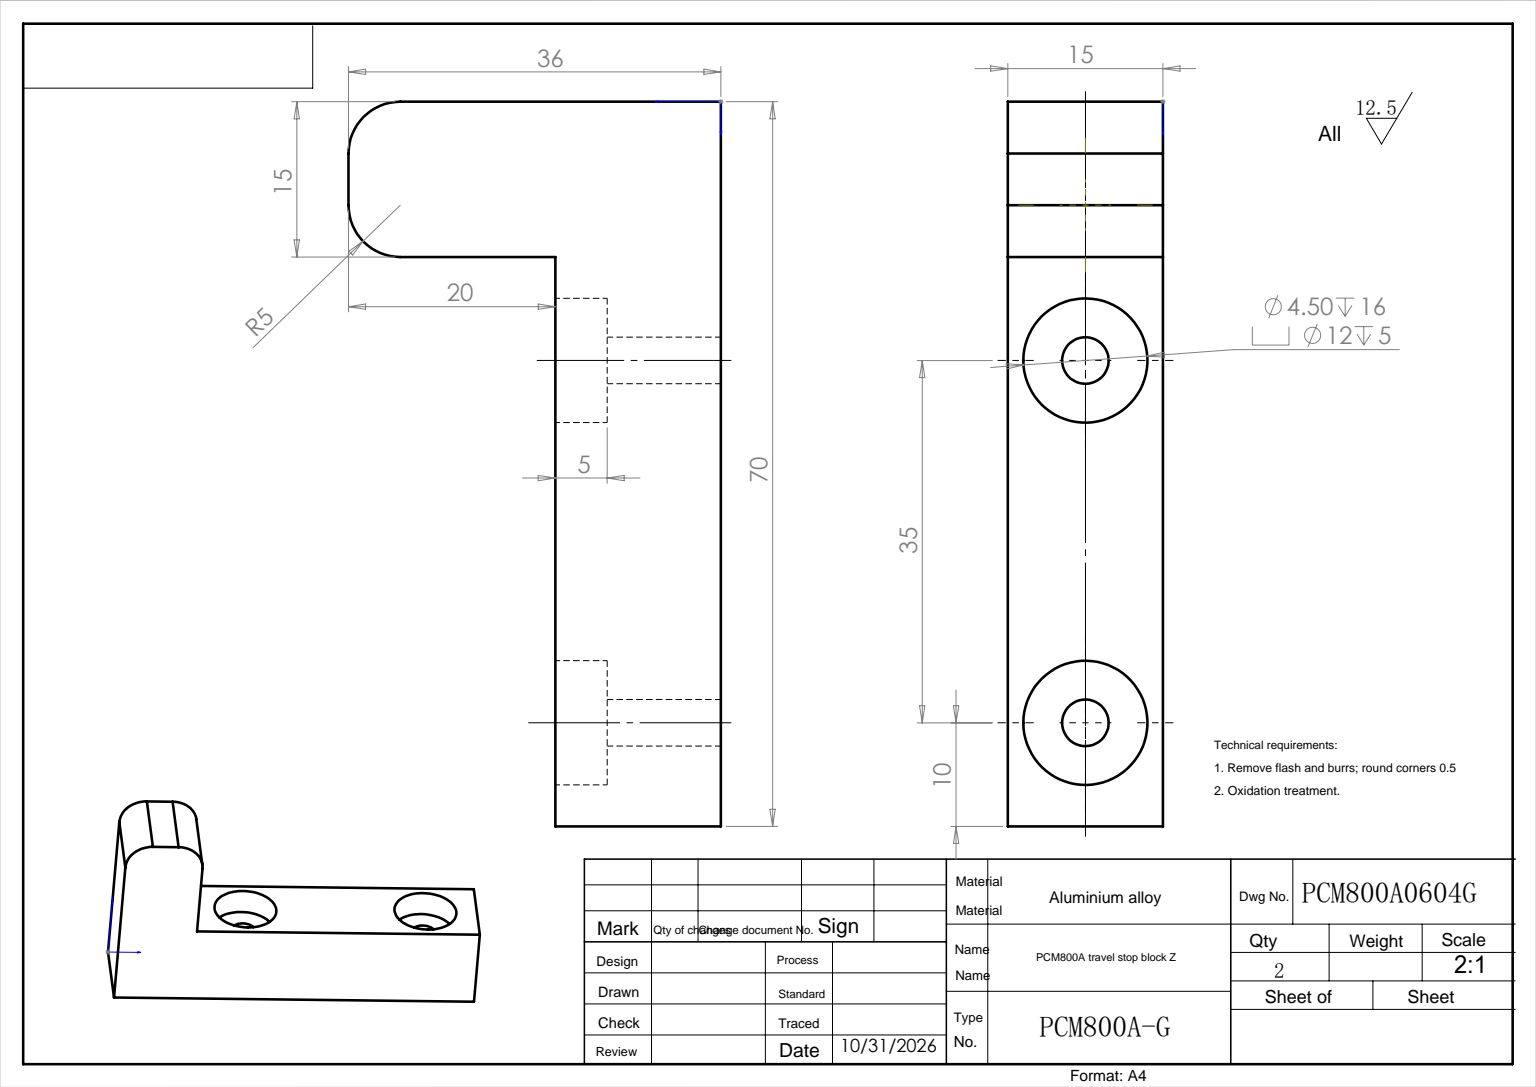
from build123d import *

# Parameters (mm, degrees)
EXTRUDE_1_DEPTH           = 15
FILLET_1_R                = 5
HOLE_WIZARD_1_D           = 4.5
HOLE_WIZARD_1_DEPTH       = 100
HOLE_WIZARD_1_CBORE_D     = 12
HOLE_WIZARD_1_CBORE_DEPTH = 5


with BuildPart() as part:
    # 草图1 → 凸台-拉伸1 (new body)
    with BuildSketch(Plane.XY):
        Polygon((0, 0), (70, 0), (70, 16), (15, 16), (15, 36), (0, 36), (0, 16), align=None)
    extrude(amount=EXTRUDE_1_DEPTH)

    # 圆角1
    fillet_1_edges = [part.edges().sort_by_distance(p)[0] for p in [
        (0, 36, 7.5),
        (15, 36, 7.5),
    ]]
    fillet(fillet_1_edges, radius=FILLET_1_R)

    # 孔1
    with Locations(Plane(origin=(0, 16, 0), x_dir=(-1, 0, 0), z_dir=(0, 1, 0))):
        with Locations((-25, 7.5), (-60, 7.5)):
            CounterBoreHole(HOLE_WIZARD_1_D / 2, HOLE_WIZARD_1_CBORE_D / 2, HOLE_WIZARD_1_CBORE_DEPTH, depth=HOLE_WIZARD_1_DEPTH)


solid = part.part
